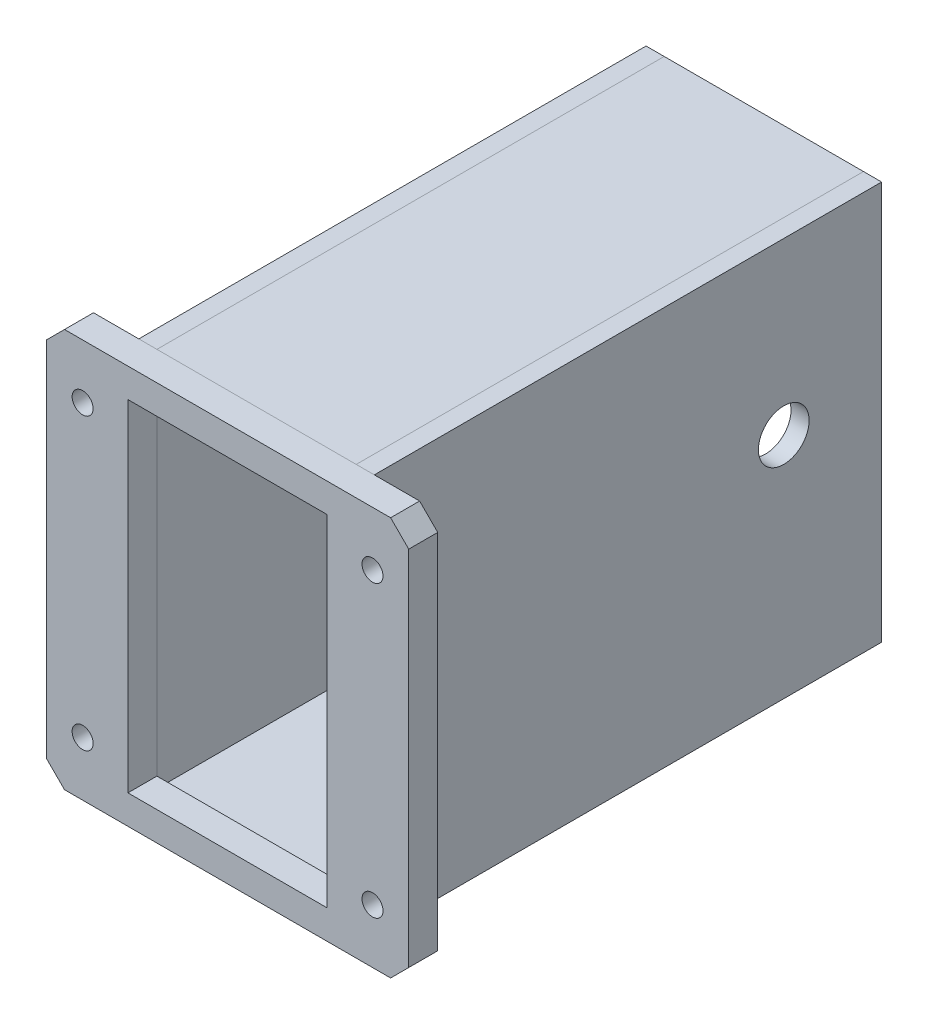
from build123d import *

# Parameters (mm, degrees)
SKETCH1_W                     = 100
SKETCH1_H                     = 110
BOSS_EXTRUDE1_DEPTH           = 8
SKETCH2_W                     = 55
SKETCH2_H                     = 94
CUT_EXTRUDE1_DEPTH            = 8
SKETCH3_W                     = 5
SKETCH3_H                     = 110
BOSS_EXTRUDE2_DEPTH           = 140
BOSS_EXTRUDE2_2_DEPTH         = 140
SKETCH4_W                     = 55
SKETCH4_H                     = 5
BOSS_EXTRUDE3_DEPTH           = 140
BOSS_EXTRUDE3_2_DEPTH         = 140
CHAMFER1_SIZE                 = 5
SKETCH6_W                     = 2.9
SKETCH6_H                     = 148
M5_CLEARANCE_HOLE1_AT_2_COUNT = 2
M5_CLEARANCE_HOLE1_AT_2_PITCH = 80
M5_CLEARANCE_HOLE1_AT_3_COUNT = 2
M5_CLEARANCE_HOLE1_AT_3_PITCH = 113.13708499
M5_CLEARANCE_HOLE1_AT_4_COUNT = 2
M5_CLEARANCE_HOLE1_AT_4_PITCH = 80
SKETCH7_R                     = 7
CUT_EXTRUDE2_DEPTH            = 172.555384643


with BuildPart() as part:
    # Sketch1 → Boss-Extrude1 (new body)
    with BuildSketch(Plane.XY):
        Rectangle(SKETCH1_W, SKETCH1_H)
    extrude(amount=BOSS_EXTRUDE1_DEPTH)

    # Sketch2 → Cut-Extrude1 (cut)
    with BuildSketch(Plane.XY.offset(8)):
        Rectangle(SKETCH2_W, SKETCH2_H)
    extrude(amount=-CUT_EXTRUDE1_DEPTH, mode=Mode.SUBTRACT)

    # Chamfer1
    chamfer1_edges = [part.edges().sort_by_distance(p)[0] for p in [
        (50, -55, 4),
        (-50, -55, 4),
        (-50, 55, 4),
        (50, 55, 4),
    ]]
    chamfer(chamfer1_edges, length=CHAMFER1_SIZE)

    # Sketch6 → M5 Clearance Hole1 (revolve, cut)
    with BuildSketch(Plane(origin=(-40, 40, 8), x_dir=(0, -1, 0), z_dir=(1, 0, 0))):
        with Locations((1.45, 74)):
            Rectangle(SKETCH6_W, SKETCH6_H)
    m5_clearance_hole1 = revolve(axis=Axis((-40, 40, 14.35), (0, 0, -1)), mode=Mode.SUBTRACT)

    # M5 Clearance Hole1 at 2: M5 Clearance Hole1 ×2
    with Locations(*[(0, -i * M5_CLEARANCE_HOLE1_AT_2_PITCH, 0) for i in range(1, M5_CLEARANCE_HOLE1_AT_2_COUNT)]):
        add(m5_clearance_hole1, mode=Mode.SUBTRACT)

    # M5 Clearance Hole1 at 3: M5 Clearance Hole1 ×2
    with Locations(*[Vector(0.7071067811865476, -0.7071067811865476, 0) * (i * M5_CLEARANCE_HOLE1_AT_3_PITCH) for i in range(1, M5_CLEARANCE_HOLE1_AT_3_COUNT)]):
        add(m5_clearance_hole1, mode=Mode.SUBTRACT)

    # M5 Clearance Hole1 at 4: M5 Clearance Hole1 ×2
    with Locations(*[(i * M5_CLEARANCE_HOLE1_AT_4_PITCH, 0, 0) for i in range(1, M5_CLEARANCE_HOLE1_AT_4_COUNT)]):
        add(m5_clearance_hole1, mode=Mode.SUBTRACT)


with BuildPart() as body_2:
    # Sketch3 → Boss-Extrude2 (new body)
    with BuildSketch(Plane(origin=(0, 0, 0), x_dir=(-1, 0, 0), z_dir=(0, 0, -1))):
        with Locations((-30, 0)):
            Rectangle(SKETCH3_W, SKETCH3_H)
    extrude(amount=BOSS_EXTRUDE2_DEPTH)


with BuildPart() as body_3:
    # Sketch3 → Boss-Extrude2 2 (new body)
    with BuildSketch(Plane(origin=(0, 0, 0), x_dir=(-1, 0, 0), z_dir=(0, 0, -1))):
        with Locations((30, 0)):
            Rectangle(SKETCH3_W, SKETCH3_H)
    extrude(amount=BOSS_EXTRUDE2_2_DEPTH)


with BuildPart() as body_4:
    # Sketch4 → Boss-Extrude3 (new body)
    with BuildSketch(Plane(origin=(0, 0, 0), x_dir=(-1, 0, 0), z_dir=(0, 0, -1))):
        with Locations((0, 52.5)):
            Rectangle(SKETCH4_W, SKETCH4_H)
    extrude(amount=BOSS_EXTRUDE3_DEPTH)


with BuildPart() as body_5:
    # Sketch4 → Boss-Extrude3 2 (new body)
    with BuildSketch(Plane(origin=(0, 0, 0), x_dir=(-1, 0, 0), z_dir=(0, 0, -1))):
        with Locations((0, -52.5)):
            Rectangle(SKETCH4_W, SKETCH4_H)
    extrude(amount=BOSS_EXTRUDE3_2_DEPTH)


with BuildPart() as cut_extrude2_tool:
    # Sketch7 → Cut-Extrude2 (new, through all)
    with BuildSketch(Plane(origin=(32.5, 0, 0), x_dir=(0, 0, -1), z_dir=(1, 0, 0))):
        with Locations(Location((113, 8, 0), (0, 0, 90))):
            Circle(SKETCH7_R)
    extrude(amount=-CUT_EXTRUDE2_DEPTH)


with BuildPart() as body_2_1:
    add(body_2.part)

    # Cut-Extrude2: cut by cut_extrude2_tool
    add(cut_extrude2_tool.part, mode=Mode.SUBTRACT)


with BuildPart() as body_3_1:
    add(body_3.part)

    # Cut-Extrude2: cut by cut_extrude2_tool
    add(cut_extrude2_tool.part, mode=Mode.SUBTRACT)


solid = Compound([part.part, body_4.part, body_5.part, body_2_1.part, body_3_1.part])
